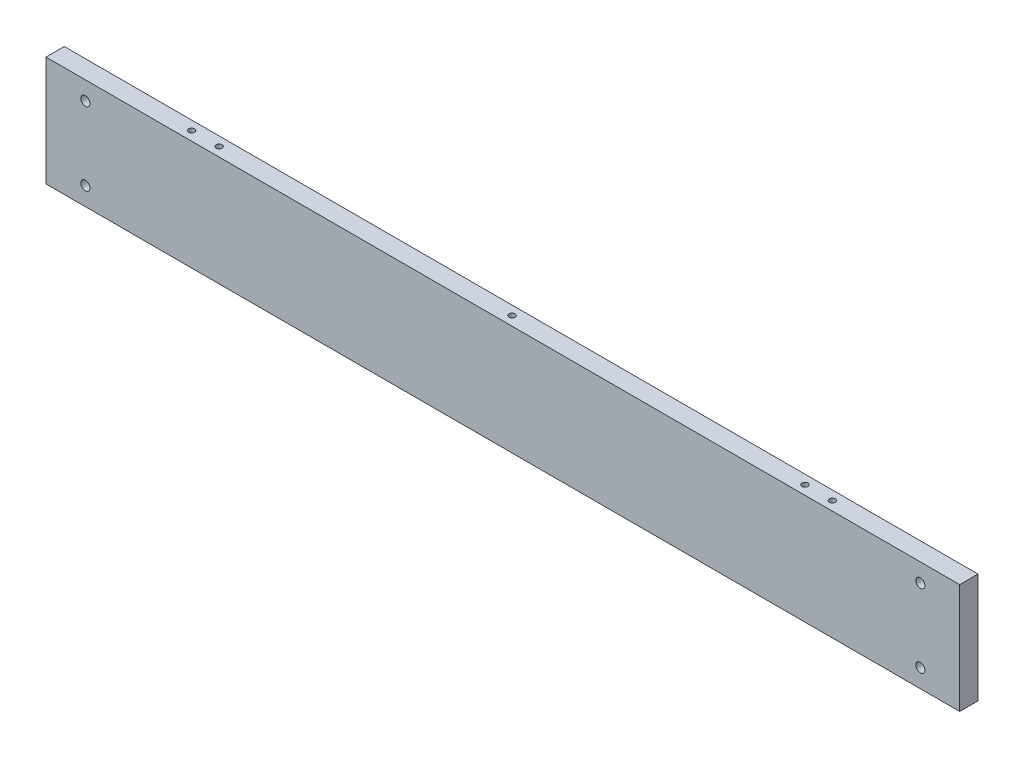
from build123d import *

# Parameters (mm, degrees)
SKETCH_1_W             = 499
SKETCH_1_H             = 10
EXTRUDE_1_DEPTH        = 60
HOLE_WIZARD_M5_1_D     = 4.2
HOLE_WIZARD_M5_1_DEPTH = 12.4
HOLE_WIZARD_M5_1_TIP   = 1.2618073
HOLE_WIZARD_M6_1_D     = 5
HOLE_WIZARD_M4_1_D     = 3.3
HOLE_WIZARD_M4_1_DEPTH = 10.1
HOLE_WIZARD_M4_1_TIP   = 0.991420021


with BuildPart() as part:
    # 草图1 → 凸台-拉伸1 (new body)
    with BuildSketch(Plane(origin=(0, 0, 0), x_dir=(1, 0, 0), z_dir=(0, 1, 0))):
        Rectangle(SKETCH_1_W, SKETCH_1_H)
    extrude(amount=EXTRUDE_1_DEPTH)

    # M5 螺纹孔1
    with Locations(Plane(origin=(0, 0, 0), x_dir=(-1, 0, 0), z_dir=(0, -1, 0))):
        with Locations((-220, 0), (-110, 0), (0, 0), (110, 0), (220, 0)):
            Hole(HOLE_WIZARD_M5_1_D / 2, depth=HOLE_WIZARD_M5_1_DEPTH)
            with Locations((0, 0, -(HOLE_WIZARD_M5_1_DEPTH + HOLE_WIZARD_M5_1_TIP / 2))):  # 118° drill point
                Cone(0, HOLE_WIZARD_M5_1_D / 2, HOLE_WIZARD_M5_1_TIP, mode=Mode.SUBTRACT)

    # M6 螺纹孔1 (through all)
    with Locations(Plane.XY.offset(5)):
        with Locations((228, 50), (228, 10), (-228, 10), (-228, 50)):
            Hole(HOLE_WIZARD_M6_1_D / 2)

    # M4 螺纹孔1
    with Locations(Plane(origin=(0, 60, 0), x_dir=(1, 0, 0), z_dir=(0, 1, 0))):
        with Locations((0, 0), (-175, 0), (175, 0), (-160, 0), (160, 0)):
            Hole(HOLE_WIZARD_M4_1_D / 2, depth=HOLE_WIZARD_M4_1_DEPTH)
            with Locations((0, 0, -(HOLE_WIZARD_M4_1_DEPTH + HOLE_WIZARD_M4_1_TIP / 2))):  # 118° drill point
                Cone(0, HOLE_WIZARD_M4_1_D / 2, HOLE_WIZARD_M4_1_TIP, mode=Mode.SUBTRACT)


solid = part.part
